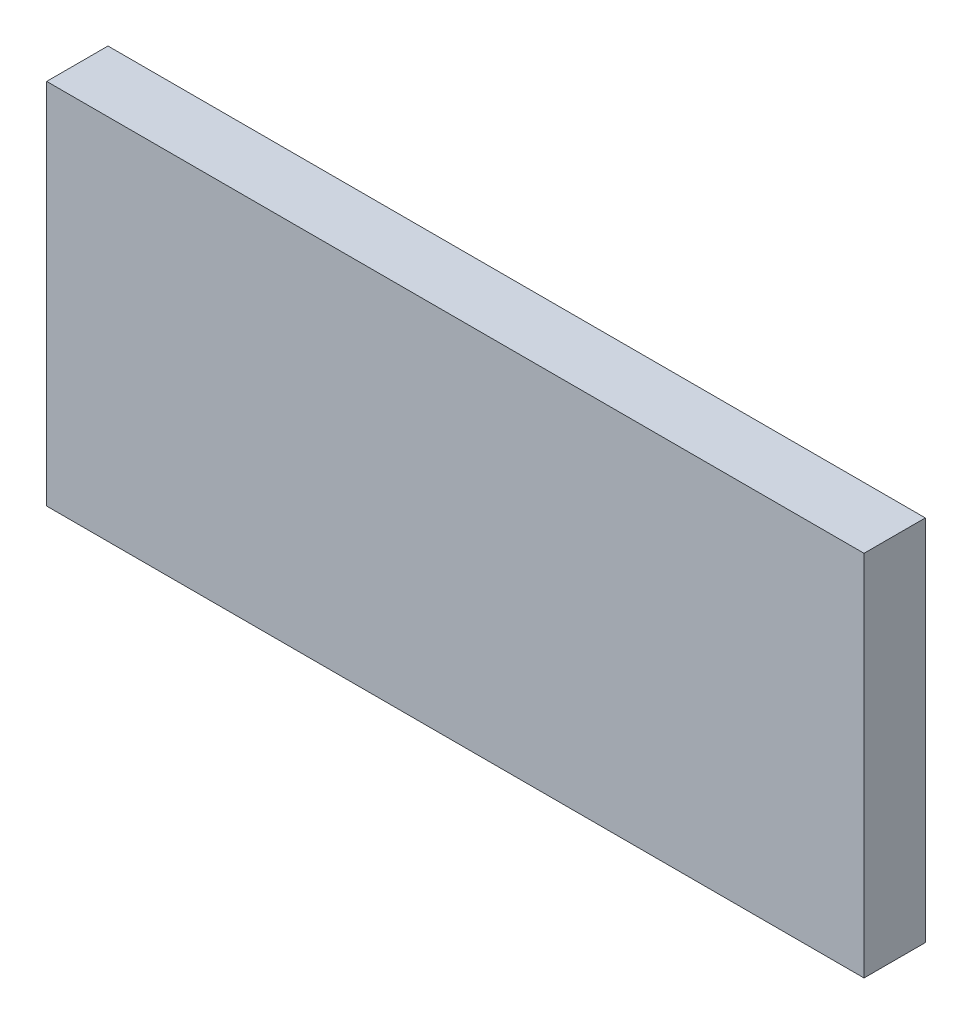
from build123d import *

# Parameters (mm, degrees)
SKETCH1_W           = 200
SKETCH1_H           = 90
BOSS_EXTRUDE1_DEPTH = 7.5


with BuildPart() as part:
    # Sketch1 → Boss-Extrude1 (new, symmetric)
    with BuildSketch(Plane.XY):
        Rectangle(SKETCH1_W, SKETCH1_H)
    extrude(amount=BOSS_EXTRUDE1_DEPTH, both=True)


solid = part.part
